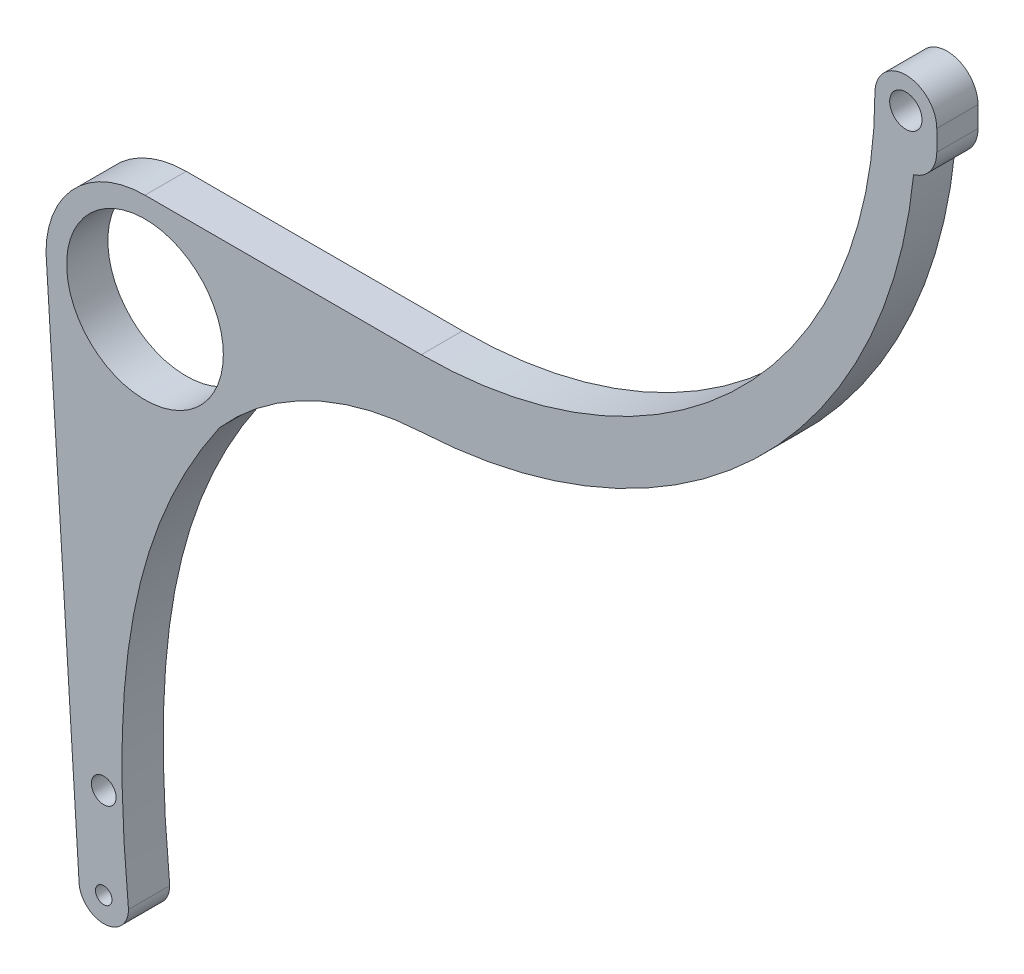
SolidWorks part; units mm, degrees
ref_plane "前视基准面" through (0, 0, 0) normal (0, 0, 1) x (1, 0, 0)
ref_plane "上视基准面" through (0, 0, 0) normal (0, 1, 0) x (1, 0, 0)
ref_plane "右视基准面" through (0, 0, 0) normal (1, 0, 0) x (0, 0, -1)
other "Configuration Table"
sketch "草图1" plane through (0, 0, 0) normal (0, 0, 1) x (1, 0, 0)
  line L0 (-60.8711, 0) -> (72.3657, 0) construction
  line L1 (-84.052, 128) -> (106.5467, 128) construction
  line L2 (0, 22) -> (0, -18.0859) construction
  line L3 (0, -18.0859) -> (10, -18.0859) construction
  line L4 (10, -18.0859) -> (10, 407.7959) construction
  line L5 (-9, 59.8208) -> (-9, -18.0859) construction
  line L6 (-14, 128) -> (-6, 0)
  line L7 (-176.4012, 262) -> (270.3663, 262) construction
  line L8 (77, 485.9134) -> (77, 110.3328) construction
  line L9 (10, 152) -> (77, 152)
  line L10 (187, 262) -> (194.5, 262) construction
  line L11 (202, 262) -> (202, 257)
  line L12 (202, 257) -> (194.1788, 257) construction
  line L13 (70.6056, 267.7759) -> (70.6056, 254.1409) construction
  line L14 (4.2515, 65.8248) -> (157.9856, 65.8248) construction
  line L15 (80.543, 130.5208) -> (80.543, 47.5555) construction
  line L16 (4.7446, 112.1309) -> (49.2871, 112.1309) construction
  circle A0 centre (0, 0) radius 2
  arc A1 (-6, 0) -> (6, 0) centre (0, 0) ccw
  circle A2 centre (10, 128) radius 19
  arc A3 (10, 152) -> (-14, 128) centre (10, 128) ccw
  circle A4 centre (77, 262) radius 115 construction
  arc A5 (77, 152) -> (187, 262) centre (77, 262) ccw
  arc A6 (202, 262) -> (187, 262) centre (194.5, 262) ccw
  arc A9 (196.3799, 249.4949) -> (202, 257) centre (194.1788, 257) ccw
  arc A10 (77, 135.7674) -> (28.0048, 112.1309) centre (80.543, 65.8248) ccw
  arc A11 (77, 135.7674) -> (196.3799, 249.4949) centre (70.6056, 262) ccw
  circle A12 centre (194.5, 262) radius 3.919
  circle A13 centre (0, 22) radius 3
  spline S0 degree 3 poles (6, 0) (1.5887, 45.6809) (5.6041, 79.6432) (28.0048, 112.1309) knots 0 0 0 0 0.788155 0.788155 0.788155 0.788155
  dimension "D1" = 4
  dimension "D2" = 12
  dimension "D5" = 19
  dimension "D6" = 134
  dimension "D8" = 230
  dimension "D9" = 6.3944
  dimension "D10" = 62.1752
  dimension "D12" = 15.8691
  dimension "D3" = 128
  dimension "D4" = 9
  dimension "D7" = 67
  dimension "D11" = 70.543
  dimension "D13" = 22
sketch "草图3" plane through (0, 0, 0) normal (0, 0, 1) x (1, 0, 0)
extrude "凸台-拉伸3" add sketch "草图1" along normal blind 10
